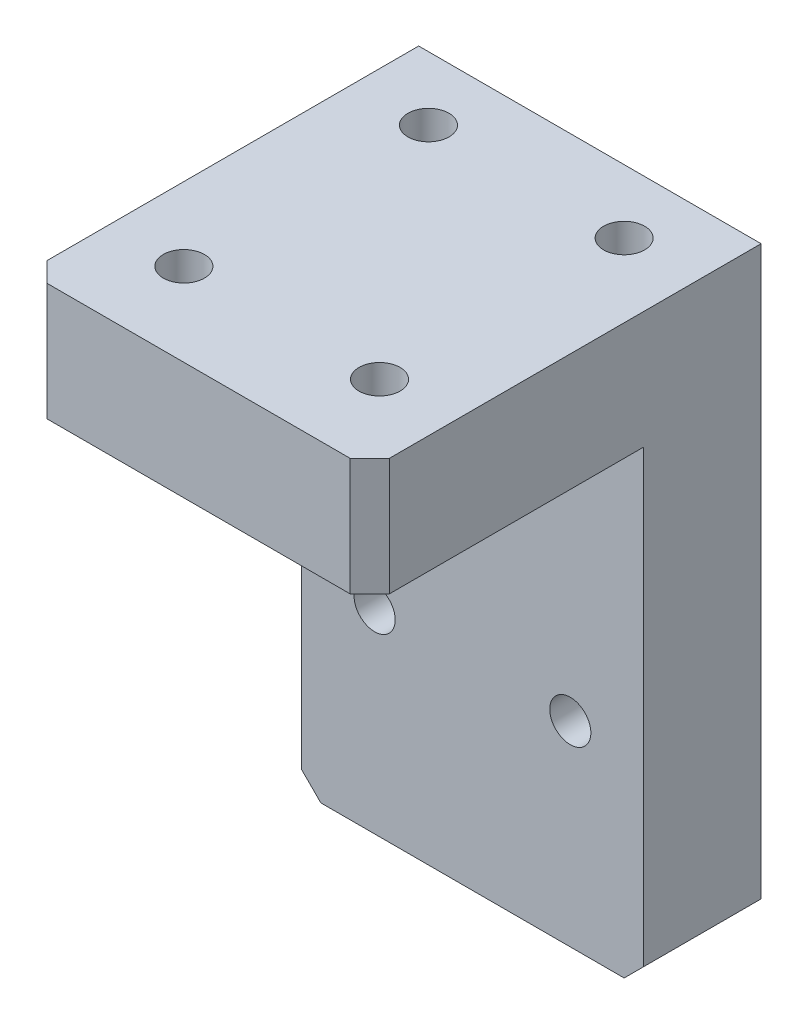
SolidWorks part; units mm, degrees
ref_plane "前视基准面" through (0, 0, 0) normal (0, 0, 1) x (1, 0, 0)
ref_plane "上视基准面" through (0, 0, 0) normal (0, 1, 0) x (1, 0, 0)
ref_plane "右视基准面" through (0, 0, 0) normal (1, 0, 0) x (0, 0, -1)
sketch "草图1" plane through (0, 0, 0) normal (0, 0, 1) x (1, 0, 0)
  line L1 (-17.5, -30) -> (17.5, -30)
  line L2 (-17.5, -30) -> (-17.5, 30)
  line L3 (-17.5, 30) -> (17.5, 30)
  line L4 (17.5, -30) -> (17.5, 30)
  line L5 (-17.5, -30) -> (17.5, 30) construction
  line L6 (-17.5, 30) -> (17.5, -30) construction
  point P0 (0, 0)
  dimension "D1" = 35
  dimension "D2" = 60
extrude "凸台-拉伸1" add sketch "草图1" along normal blind 12 contours L3 L4 L1 L2
chamfer "倒角1" distance 2 angle 45
sketch "草图4" plane through (-17.5, 0, 0) normal (-1, 0, 0) x (0, 0, 1)
  line L1 (12, 30) -> (40, 30)
  line L2 (12, 30) -> (12, 18)
  line L3 (12, 18) -> (40, 18)
  line L4 (40, 30) -> (40, 18)
  line L6 (12, -28) -> (12, 30) construction
  line L7 (12, 30) -> (0, 30) construction
  dimension "D1" = 28
  dimension "D2" = 12
extrude "凸台-拉伸2" add sketch "草图4" against normal up to surface (35 mm away)
sketch "草图7" plane through (0, 0, 0) normal (0, 0, -1) x (-1, 0, 0)
  point P11 (-10, -10)
  point P14 (10, -10)
hole_wizard "M5 螺纹孔1" positions "草图7" profile "草图6" tap size "M5" standard "GB"
sketch "草图6" plane through (10, -10, 0) normal (1, 0, 0) x (0, 1, 0)
  line L0 (0, 0) -> (0, 40)
  line L1 (0, 40) -> (2.1, 40)
  line L2 (2.1, 40) -> (2.1, 0)
  line L5 (2.1, 0) -> (0, 0)
  line L11 (0, -6.35) -> (0, 107.95) construction
  dimension "通孔螺纹孔钻头直径" = 4.2
  dimension "通孔螺纹孔钻头深度" = 40
cosmetic thread "孔螺纹线1" parameters "D2"=5
cosmetic thread "孔螺纹线8" parameters "D2"=5
chamfer "倒角2" distance 2 angle 45
sketch "草图10" plane through (0, 30, 0) normal (0, 1, 0) x (1, 0, 0)
  line L0 (17.5, -19) -> (-35.1832, -19) construction
  line L1 (17.5, -38) -> (17.5, 0) construction
  line L3 (0, -49.559) -> (0, 8.1698) construction
  point P0 (-10, -6.5)
  point P2 (10, -6.5)
  point P4 (-10, -31.5)
  point P6 (10, -31.5)
  dimension "D1" = 25
  dimension "D2" = 20
hole_wizard "M5 螺纹孔2" positions "草图10" profile "草图9" tap size "M5" standard "GB"
sketch "草图9" plane through (-10, 30, 6.5) normal (1, 0, 0) x (0, 0, 1)
  line L0 (0, 0) -> (0, 13.6618)
  line L1 (0, 13.6618) -> (2.1, 12.4)
  line L2 (2.1, 12.4) -> (2.1, 0)
  line L5 (2.1, 0) -> (0, 0)
  line L10 (0, 13.6618) -> (-2.1, 12.4) construction
  line L11 (0, -6.35) -> (0, 107.95) construction
  dimension "螺纹孔钻头直径" = 4.2
  dimension "螺纹孔钻头深度" = 12.4
  dimension "导头角度" = 118
cosmetic thread "孔螺纹线3" parameters "D1"=10, "D2"=5
cosmetic thread "孔螺纹线4" parameters "D1"=10, "D2"=5
cosmetic thread "孔螺纹线5" parameters "D1"=10, "D2"=5
cosmetic thread "孔螺纹线6" parameters "D1"=10, "D2"=5
